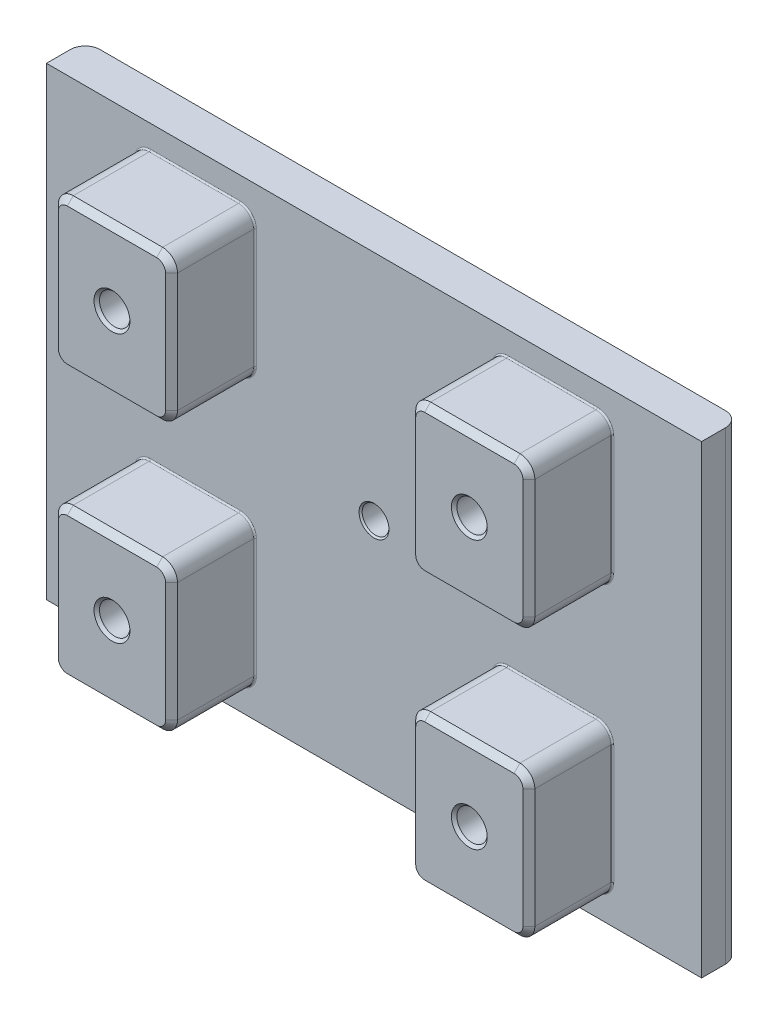
SolidWorks part; units mm, degrees
material "ZCuAL10Fe3#"
ref_plane "前视基准面" through (0, 0, 0) normal (0, 0, 1) x (1, 0, 0)
ref_plane "上视基准面" through (0, 0, 0) normal (0, 1, 0) x (1, 0, 0)
ref_plane "右视基准面" through (0, 0, 0) normal (1, 0, 0) x (0, 0, -1)
sketch "草图1" plane through (0, 0, 0) normal (0, 0, 1) x (1, 0, 0)
  line L1 (0, 0) -> (220, 0)
  line L2 (0, 0) -> (0, -156)
  line L3 (0, -156) -> (220, -156)
  line L4 (220, 0) -> (220, -156)
  dimension "D1" = 156
  dimension "D2" = 220
extrude "凸台-拉伸1" add sketch "草图1" along normal blind 13
sketch "草图2" plane through (0, 0, 13) normal (0, 0, 1) x (1, 0, 0)
  line L0 (0, -78) -> (220, -78) construction
  line L1 (0, 0) -> (0, -156) construction
  line L2 (220, -156) -> (220, 0) construction
  line L3 (110, -33) -> (110, -78) construction
  line L4 (50, -33) -> (170, -33) construction
  line L5 (50, -33) -> (50, -123) construction
  line L6 (50, -123) -> (170, -123) construction
  line L7 (170, -33) -> (170, -123) construction
  line L8 (50, -33) -> (170, -123) construction
  line L9 (50, -123) -> (170, -33) construction
  line L10 (30, -8) -> (70, -8)
  line L11 (30, -8) -> (30, -58)
  line L12 (30, -58) -> (70, -58)
  line L13 (70, -8) -> (70, -58)
  line L14 (30, -8) -> (70, -58) construction
  line L15 (30, -58) -> (70, -8) construction
  line L16 (150, -8) -> (150, -58)
  line L17 (190, -58) -> (150, -58)
  line L18 (190, -8) -> (190, -58)
  line L19 (190, -8) -> (150, -8)
  line L20 (190, -148) -> (190, -98)
  line L21 (190, -98) -> (150, -98)
  line L22 (150, -148) -> (150, -98)
  line L23 (190, -148) -> (150, -148)
  line L24 (30, -148) -> (70, -148)
  line L25 (30, -98) -> (70, -98)
  line L26 (70, -148) -> (70, -98)
  line L27 (30, -148) -> (30, -98)
  circle A0 centre (50, -33) radius 20 construction
  circle A1 centre (50, -123) radius 20 construction
  circle A2 centre (170, -123) radius 20 construction
  circle A3 centre (170, -33) radius 20 construction
  point P6 (110, -78)
  dimension "D4" = 40
  dimension "D1" = 120
  dimension "D2" = 90
  dimension "D3" = 50
  dimension "D5" = 50
  dimension "D6" = 40
extrude "凸台-拉伸2" add sketch "草图2" along normal blind 28
fillet "圆角1" radius 5 2 edges at (0, -78, 0) (220, -78, 0)
sketch "草图8" plane through (0, 0, 41) normal (0, 0, 1) x (1, 0, 0)
  line L0 (50, -8) -> (50, -58) construction
  line L1 (70, -8) -> (30, -8) construction
  line L2 (30, -58) -> (70, -58) construction
  line L3 (50, -58) -> (50, -98) construction
  line L4 (70, -98) -> (30, -98) construction
  line L5 (50, -98) -> (50, -148) construction
  line L6 (30, -148) -> (70, -148) construction
  line L7 (170, -8) -> (170, -58) construction
  line L8 (190, -8) -> (150, -8) construction
  line L9 (150, -58) -> (190, -58) construction
  line L10 (170, -58) -> (170, -98) construction
  line L11 (190, -98) -> (150, -98) construction
  line L12 (170, -98) -> (170, -148) construction
  line L13 (150, -148) -> (190, -148) construction
  line L14 (50, -33) -> (170, -33) construction
  line L15 (50, -123) -> (170, -123) construction
hole_wizard "M12 螺纹孔1" positions "3D草图2" profile "草图9" tap size "M12" standard "GB"
sketch3d "3D草图2"
  point P0 (50, -33, 41)
  point P3 (170, -33, 41)
  point P6 (170, -123, 41)
  point P9 (50, -123, 41)
sketch "草图9" plane through (50, -33, 41) normal (1, 0, 0) x (0, -1, 0)
  line L0 (0, 0) -> (0, 33.0644)
  line L1 (0, 33.0644) -> (5.1, 30)
  line L2 (5.1, 30) -> (5.1, 0.925)
  line L3 (5.1, 0.925) -> (6.025, 0)
  line L5 (6.025, 0) -> (0, 0)
  line L6 (-5.1, 0.925) -> (-6.025, 0) construction
  line L10 (0, 33.0644) -> (-5.1, 30) construction
  line L11 (0, -6.35) -> (0, 107.95) construction
  dimension "螺纹孔钻头直径" = 10.2
  dimension "螺纹孔钻头深度" = 30
  dimension "近端锥形沉头孔直径" = 12.05
  dimension "近端锥形沉头孔角度" = 90
  dimension "导头角度" = 118
cosmetic thread "孔螺蚊线1" parameters "D1"=24, "D2"=12
cosmetic thread "孔螺蚊线2" parameters "D1"=24, "D2"=12
cosmetic thread "孔螺蚊线3" parameters "D1"=24, "D2"=12
cosmetic thread "孔螺蚊线4" parameters "D1"=24, "D2"=12
sketch "草图10" plane through (0, 0, 13) normal (0, 0, 1) x (1, 0, 0)
  line L0 (110, 0) -> (110, -156) construction
  line L1 (220, 0) -> (0, 0) construction
  line L2 (0, -156) -> (220, -156) construction
  line L3 (110, -78) -> (148.6826, -78) construction
hole_wizard "M10x1.0 螺纹孔1" positions "3D草图3" profile "草图11" tap size "M10x1.0" standard "GB"
sketch3d "3D草图3"
  point P0 (110, -78, 13)
sketch "草图11" plane through (110, -78, 13) normal (1, 0, 0) x (0, -1, 0)
  line L0 (0, 0) -> (0, 27.7039)
  line L1 (0, 27.7039) -> (4.5, 25)
  line L2 (4.5, 25) -> (4.5, 0.525)
  line L3 (4.5, 0.525) -> (5.025, 0)
  line L5 (5.025, 0) -> (0, 0)
  line L6 (-4.5, 0.525) -> (-5.025, 0) construction
  line L10 (0, 27.7039) -> (-4.5, 25) construction
  line L11 (0, -6.35) -> (0, 107.95) construction
  dimension "螺纹孔钻头直径" = 9
  dimension "螺纹孔钻头深度" = 25
  dimension "近端锥形沉头孔直径" = 10.05
  dimension "近端锥形沉头孔角度" = 90
  dimension "导头角度" = 118
cosmetic thread "孔螺蚊线5" parameters "D1"=8.5, "D2"=10
fillet "圆角2" radius 5 16 edges at (70, -98, 27) (30, -98, 27) (30, -148, 27) (70, -148, 27) (150, -148, 27) (190, -148, 27) (190, -98, 27) (150, -98, 27) (150, -8, 27) (190, -8, 27) (190, -58, 27) (150, -58, 27) (70, -58, 27) (30, -58, 27) (70, -8, 27) (30, -8, 27)
chamfer "倒角1" distance 2 angle 45 32 edges at (150, -123, 41) (151.4645, -146.5355, 41) (151.4645, -99.4645, 41) (170, -148, 41) (170, -98, 41) (188.5355, -146.5355, 41) (188.5355, -99.4645, 41) (190, -123, 41) (30, -123, 41) (31.4645, -146.5355, 41) (31.4645, -99.4645, 41) (50, -148, 41) (50, -98, 41) (68.5355, -146.5355, 41) (68.5355, -99.4645, 41) (70, -123, 41) (150, -33, 41) (151.4645, -56.5355, 41) (151.4645, -9.4645, 41) (170, -58, 41) (170, -8, 41) (188.5355, -56.5355, 41) (188.5355, -9.4645, 41) (190, -33, 41) (30, -33, 41) (31.4645, -56.5355, 41) (31.4645, -9.4645, 41) (50, -58, 41) (50, -8, 41) (68.5355, -56.5355, 41) (68.5355, -9.4645, 41) (70, -33, 41)
sketch "草图12" plane through (0, 0, 0) normal (0, 0, -1) x (-1, 0, 0)
  line L0 (-110, -128) -> (-110, -28) construction
  line L1 (-116, -128) -> (-116, -28)
  line L2 (-104, -128) -> (-104, -28)
  arc A0 (-116, -128) -> (-104, -128) centre (-110, -128) ccw
  arc A1 (-104, -28) -> (-116, -28) centre (-110, -28) ccw
  point P2 (-110, -78)
  dimension "D2" = 6
  dimension "D1" = 100
extrude "切除-拉伸1" cut sketch "草图12" against normal blind 1
sketch "草图13" plane through (0, 0, 0) normal (0, 0, -1) x (-1, 0, 0)
  line L0 (-185, -28) -> (-35, -28) construction
  line L1 (-185, -22) -> (-35, -22)
  line L2 (-185, -34) -> (-35, -34)
  line L3 (-110, -78) -> (-5, -78) construction
  line L4 (-5, -156) -> (-5, 0) construction
  line L5 (-185, -128) -> (-35, -128) construction
  line L6 (-185, -134) -> (-35, -134)
  line L7 (-185, -122) -> (-35, -122)
  arc A0 (-185, -22) -> (-185, -34) centre (-185, -28) ccw
  arc A1 (-35, -34) -> (-35, -22) centre (-35, -28) ccw
  arc A2 (-185, -134) -> (-185, -122) centre (-185, -128) cw
  arc A3 (-35, -122) -> (-35, -134) centre (-35, -128) cw
  point P2 (-110, -28)
  point P15 (-110, -128)
  dimension "D2" = 6
  dimension "D1" = 150
extrude "切除-拉伸2" cut sketch "草图13" against normal blind 1
fillet "圆角3" radius 0.5 32 edges at (151.4645, -9.4645, 13) (170, -8, 13) (188.5355, -9.4645, 13) (190, -33, 13) (188.5355, -56.5355, 13) (170, -58, 13) (151.4645, -56.5355, 13) (188.5355, -99.4645, 13) (190, -123, 13) (188.5355, -146.5355, 13) (170, -148, 13) (151.4645, -146.5355, 13) (150, -123, 13) (151.4645, -99.4645, 13) (68.5355, -99.4645, 13) (70, -123, 13) (68.5355, -146.5355, 13) (50, -148, 13) (31.4645, -146.5355, 13) (30, -123, 13) (31.4645, -99.4645, 13) (68.5355, -9.4645, 13) (70, -33, 13) (68.5355, -56.5355, 13) (50, -58, 13) (31.4645, -56.5355, 13) (30, -33, 13) (31.4645, -9.4645, 13) (150, -33, 13) (170, -98, 13) (50, -98, 13) (50, -8, 13)
fillet "圆角4" radius 1 4 edges at (116, -34, 0.5) (104, -34, 0.5) (104, -122, 0.5) (116, -122, 0.5)
